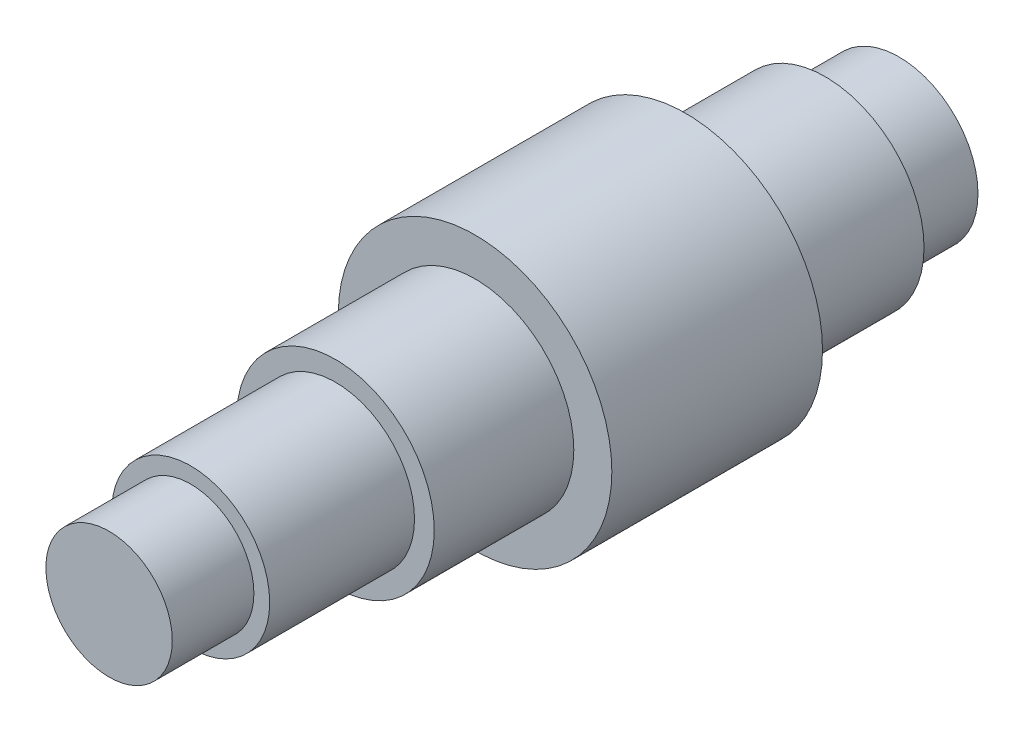
from build123d import *

# Parameters (mm, degrees)
SKETCH1_R           = 30
BOSS_EXTRUDE1_DEPTH = 28
SKETCH2_R           = 37.5
BOSS_EXTRUDE2_DEPTH = 53
SKETCH3_R           = 51.9465
BOSS_EXTRUDE3_DEPTH = 80
SKETCH4_R           = 37.5
BOSS_EXTRUDE4_DEPTH = 53
SKETCH5_R           = 30
BOSS_EXTRUDE5_DEPTH = 55
SKETCH6_R           = 24
BOSS_EXTRUDE6_DEPTH = 31


with BuildPart() as part:
    # Sketch1 → Boss-Extrude1 (new body)
    with BuildSketch(Plane.XY):
        Circle(SKETCH1_R)
    extrude(amount=BOSS_EXTRUDE1_DEPTH)

    # Sketch2 → Boss-Extrude2 (add)
    with BuildSketch(Plane.XY.offset(28)):
        Circle(SKETCH2_R)
    extrude(amount=BOSS_EXTRUDE2_DEPTH)

    # Sketch3 → Boss-Extrude3 (add)
    with BuildSketch(Plane.XY.offset(81)):
        Circle(SKETCH3_R)
    extrude(amount=BOSS_EXTRUDE3_DEPTH)

    # Sketch4 → Boss-Extrude4 (add)
    with BuildSketch(Plane.XY.offset(161)):
        Circle(SKETCH4_R)
    extrude(amount=BOSS_EXTRUDE4_DEPTH)

    # Sketch5 → Boss-Extrude5 (add)
    with BuildSketch(Plane.XY.offset(214)):
        Circle(SKETCH5_R)
    extrude(amount=BOSS_EXTRUDE5_DEPTH)

    # Sketch6 → Boss-Extrude6 (add)
    with BuildSketch(Plane.XY.offset(269)):
        Circle(SKETCH6_R)
    extrude(amount=BOSS_EXTRUDE6_DEPTH)


solid = part.part
